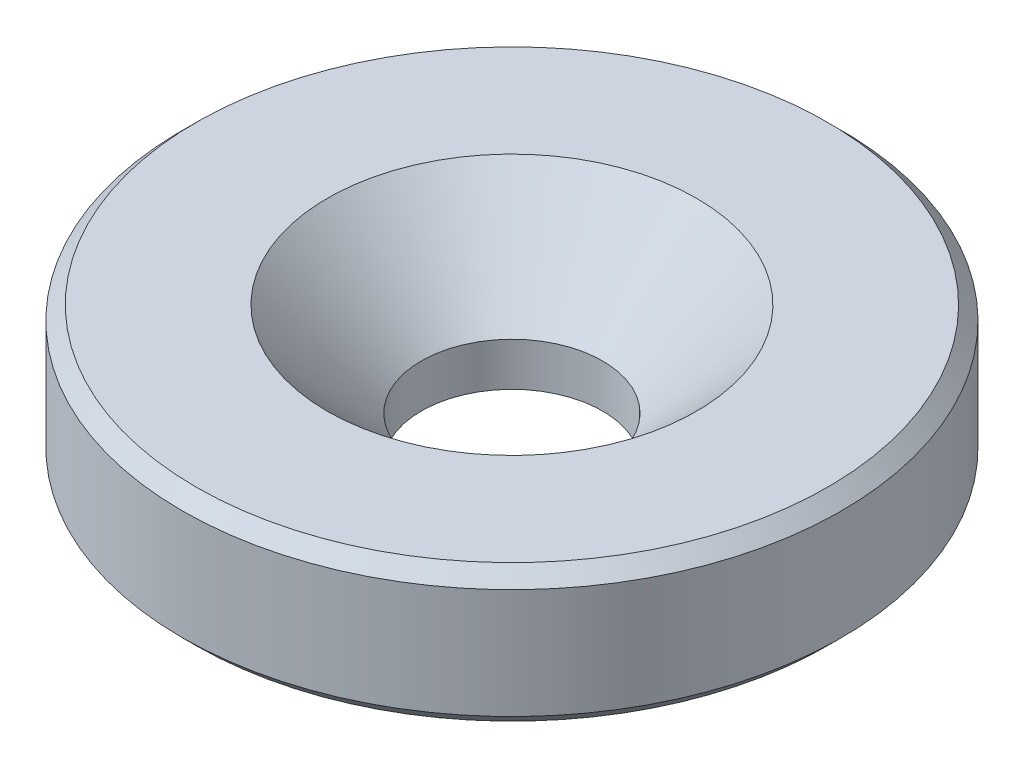
SolidWorks part; units mm, degrees
material "普通碳钢"
ref_plane "前视基准面" through (0, 0, 0) normal (0, 0, 1) x (1, 0, 0)
ref_plane "上视基准面" through (0, 0, 0) normal (0, 1, 0) x (1, 0, 0)
ref_plane "右视基准面" through (0, 0, 0) normal (1, 0, 0) x (0, 0, -1)
sketch "草图1" plane through (0, 0, 0) normal (0, 1, 0) x (1, 0, 0)
  circle A0 centre (0, 0) radius 12
  dimension "D1" = 24
extrude "凸台-拉伸1" add sketch "草图1" along normal blind 5
hole_wizard "M6 六角凹锥坑螺钉的锥形沉头孔1" positions "草图3" profile "草图2" countersink size "M6" standard "Iso" end condition through all
sketch "草图3" plane through (0, 5, 0) normal (0, 1, 0) x (1, 0, 0)
  point P0 (0, 0)
sketch "草图2" plane through (0, 5, 0) normal (1, 0, 0) x (0, 0, 1)
  line L0 (0, 0) -> (0, 5)
  line L1 (0, 5) -> (3.3, 5)
  line L2 (3.3, 5) -> (3.3, 3.42)
  line L3 (3.3, 3.42) -> (6.72, 0)
  line L5 (6.72, 0) -> (0, 0)
  line L6 (-3.3, 3.42) -> (-6.72, 0) construction
  line L11 (0, -6.35) -> (0, 107.95) construction
  dimension "通孔孔直径" = 6.6
  dimension "通孔孔深度" = 5
  dimension "近端锥形沉头孔直径" = 13.44
  dimension "近端锥形沉头孔角度" = 90
chamfer "倒角1" distance 0.5 angle 45 2 edges at (0, 0, 12) (0, 5, 12)
